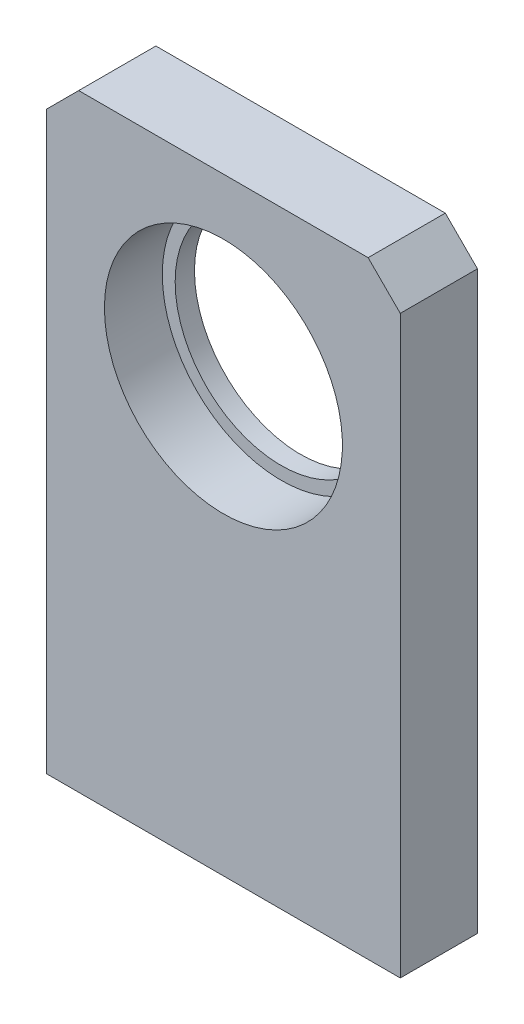
from build123d import *

# Parameters (mm, degrees)
SKETCH_1_W          = 55
SKETCH_1_H          = 94.5
EXTRUDE_1_DEPTH     = 12
CUT_EXTRUDE_4_REACH = 57.972
SKETCH_5_R          = 18.5
CHAMFER_1_SIZE      = 5
SKETCH_6_R          = 18.5
SKETCH_6_R_2        = 16.5
EXTRUDE_2_DEPTH     = 3


with BuildPart() as part:
    # 草图1 → 凸台-拉伸1 (new body)
    with BuildSketch(Plane.XY):
        Rectangle(SKETCH_1_W, SKETCH_1_H)
    extrude(amount=EXTRUDE_1_DEPTH)

    # 草图5 → 切除-拉伸4 (cut, up to next)
    with BuildSketch(Plane(origin=(0, 0, 0), x_dir=(-1, 0, 0), z_dir=(0, 0, -1)), mode=Mode.PRIVATE) as cut_extrude_4_sk1:
        with Locations((0, 20)):
            Circle(SKETCH_5_R)
    cut_extrude_4_tool1 = extrude(cut_extrude_4_sk1.sketch, amount=-CUT_EXTRUDE_4_REACH, mode=Mode.PRIVATE) & part.part
    add(cut_extrude_4_tool1.solids().sort_by_distance((0, 20, 0))[0], mode=Mode.SUBTRACT)

    # 倒角1
    chamfer_1_edges = [part.edges().sort_by_distance(p)[0] for p in [
        (-27.5, 47.25, 6),
        (27.5, 47.25, 6),
    ]]
    chamfer(chamfer_1_edges, length=CHAMFER_1_SIZE)

    # 草图6 → 凸台-拉伸2 (add)
    with BuildSketch(Plane(origin=(0, 0, 0), x_dir=(-1, 0, 0), z_dir=(0, 0, -1))):
        with Locations((0, 20)):
            Circle(SKETCH_6_R)
        with Locations((0, 20)):
            Circle(SKETCH_6_R_2, mode=Mode.SUBTRACT)
    extrude(amount=-EXTRUDE_2_DEPTH)


solid = part.part
